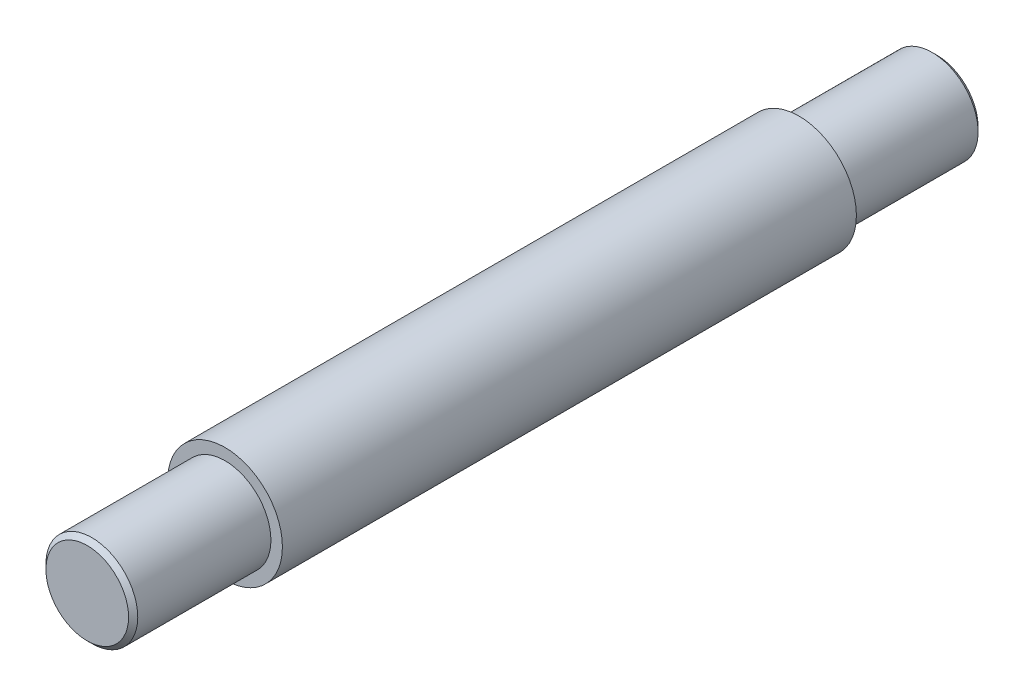
from build123d import *

# Parameters (mm, degrees)
SKETCH1_R           = 12.5
BOSS_EXTRUDE1_DEPTH = 62.5
SKETCH2_R           = 10
BOSS_EXTRUDE2_DEPTH = 30
BOSS_EXTRUDE3_START = 30
SKETCH3_R           = 10
BOSS_EXTRUDE3_DEPTH = 30
CHAMFER1_SIZE       = 1


with BuildPart() as part:
    # Sketch1 → Boss-Extrude1 (new, symmetric)
    with BuildSketch(Plane.XY):
        Circle(SKETCH1_R)
    extrude(amount=BOSS_EXTRUDE1_DEPTH, both=True)

    # Sketch2 → Boss-Extrude2 (add)
    with BuildSketch(Plane.XY.offset(62.5)):
        Circle(SKETCH2_R)
    extrude(amount=BOSS_EXTRUDE2_DEPTH)

    # Sketch3 → Boss-Extrude3 (add)
    with BuildSketch(Plane(origin=(0, 0, -62.5), x_dir=(-1, 0, 0), z_dir=(0, 0, -1)).offset(BOSS_EXTRUDE3_START)):
        with Locations(Location((0, 0, 0), (0, 0, 180))):
            Circle(SKETCH3_R)
    extrude(amount=-BOSS_EXTRUDE3_DEPTH)

    # Chamfer1
    chamfer1_edges = [part.edges().sort_by_distance(p)[0] for p in [
        (-10, 0, -92.5),
        (-10, 0, 92.5),
    ]]
    chamfer(chamfer1_edges, length=CHAMFER1_SIZE)


solid = part.part
